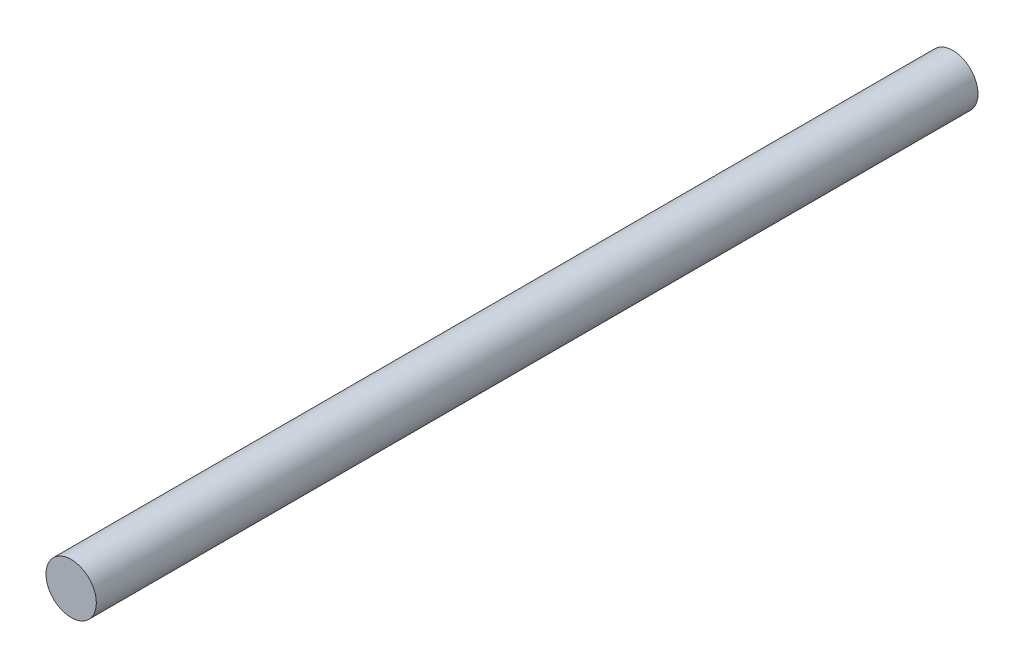
SolidWorks part; units mm, degrees
ref_plane "前视基准面" through (0, 0, 0) normal (0, 0, 1) x (1, 0, 0)
ref_plane "上视基准面" through (0, 0, 0) normal (0, 1, 0) x (1, 0, 0)
ref_plane "右视基准面" through (0, 0, 0) normal (1, 0, 0) x (0, 0, -1)
sketch "草图1" plane through (0, 0, 0) normal (0, 0, 1) x (1, 0, 0)
  circle A0 centre (0, 0) radius 4
  dimension "D1" = 8
extrude "凸台-拉伸1" add sketch "草图1" along normal mid plane 140
